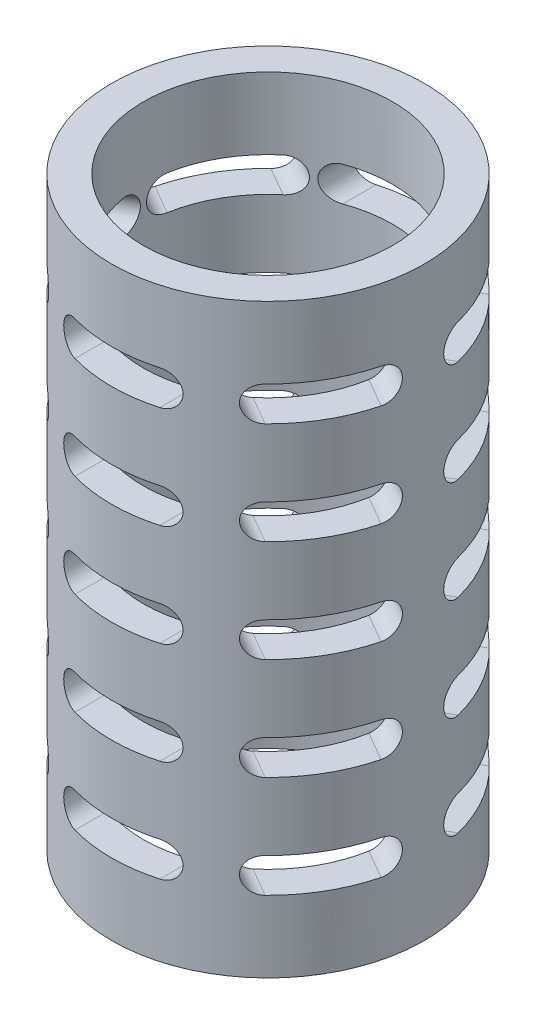
SolidWorks part; units mm, degrees
ref_plane "Front Plane" through (0, 0, 0) normal (0, 0, 1) x (1, 0, 0)
ref_plane "Top Plane" through (0, 0, 0) normal (0, 1, 0) x (1, 0, 0)
ref_plane "Right Plane" through (0, 0, 0) normal (1, 0, 0) x (0, 0, -1)
sketch "Sketch1" plane through (0, 0, 0) normal (0, 1, 0) x (1, 0, 0)
  circle A0 centre (0, 0) radius 59
  circle A1 centre (0, 0) radius 47
  dimension "D1" = 118
  dimension "D2" = 12
extrude "Boss-Extrude1" add sketch "Sketch1" along normal blind 221
sketch "Sketch2" plane through (0, 0, 0) normal (0, 0, 1) x (1, 0, 0)
  line L0 (-16, 187.5) -> (16, 187.5) construction
  line L1 (-16, 194) -> (16, 194)
  line L2 (-16, 181) -> (16, 181)
  line L3 (59, 221) -> (-59, 221) construction
  arc A0 (-16, 194) -> (-16, 181) centre (-16, 187.5) ccw
  arc A1 (16, 181) -> (16, 194) centre (16, 187.5) ccw
  point P2 (0, 187.5)
  dimension "D1" = 13
  dimension "D2" = 32
  dimension "D3" = 27
extrude "Cut-Extrude1" cut sketch "Sketch2" against normal blind 221
pattern_circular "CirPattern1" count 6 over 360 about axis through (0, 221, 0) along (0, 1, 0) of "Cut-Extrude1"
sketch "Sketch3" plane through (0, 0, 0) normal (0, 0, 1) x (1, 0, 0)
  line L0 (0, 0) -> (0, 147.2499) construction
pattern_linear "LPattern1" count 5 spacing 38.5 along (0, -1, 0) of "CirPattern1", "Cut-Extrude1"
